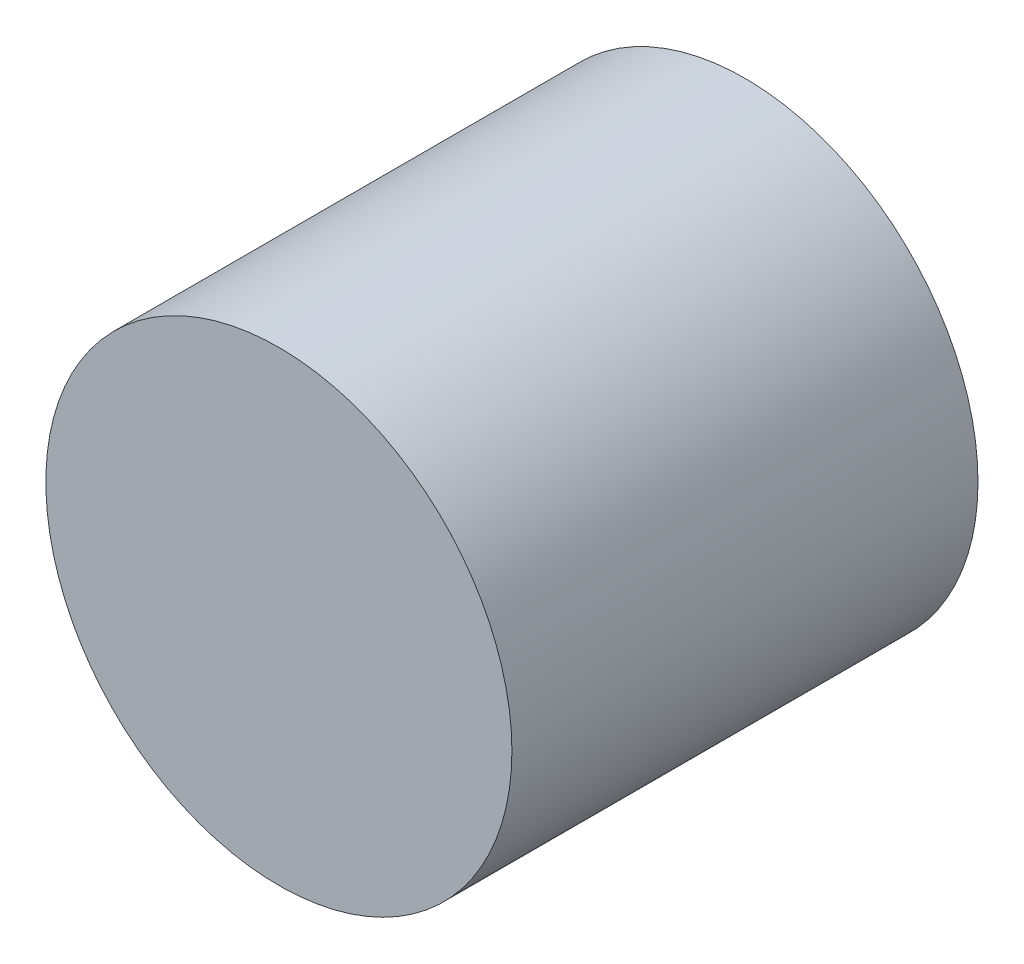
SolidWorks part; units mm, degrees
ref_plane "Front Plane" through (0, 0, 0) normal (0, 0, 1) x (1, 0, 0)
ref_plane "Top Plane" through (0, 0, 0) normal (0, 1, 0) x (1, 0, 0)
ref_plane "Right Plane" through (0, 0, 0) normal (1, 0, 0) x (0, 0, -1)
other "Configuration Table"
sketch "Sketch1" plane through (0, 0, 0) normal (0, 0, 1) x (1, 0, 0)
  line L0 (0, 18.3805) -> (0, -18.3805) construction
  circle A0 centre (0, 0) radius 9.5
  point P4 (0, 0)
  dimension "D1" = 19
extrude "Boss-Extrude1" add sketch "Sketch1" along normal blind 19
